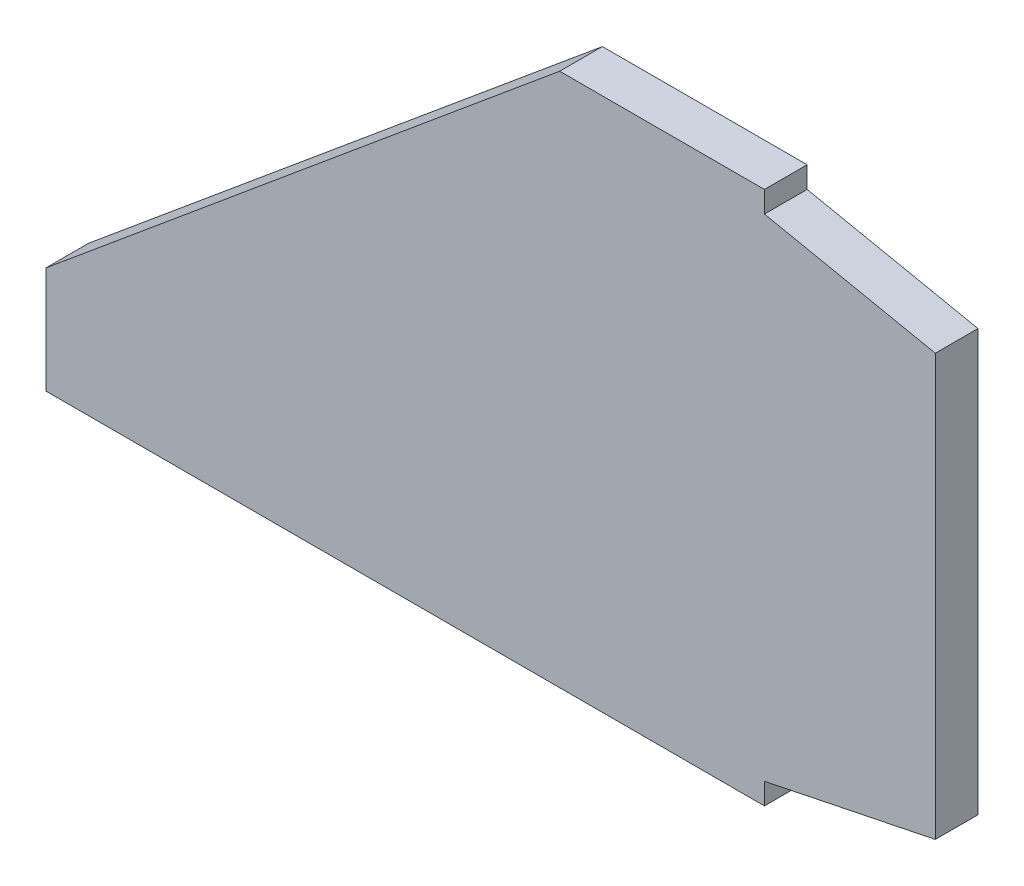
SolidWorks part; units mm, degrees
material "Q235B"
ref_plane "Front Plane" through (0, 0, 0) normal (0, 0, 1) x (1, 0, 0)
ref_plane "Top Plane" through (0, 0, 0) normal (0, 1, 0) x (1, 0, 0)
ref_plane "Right Plane" through (0, 0, 0) normal (1, 0, 0) x (0, 0, -1)
sketch "Sketch1" plane through (0, 0, 0) normal (0, 0, 1) x (1, 0, 0)
  line L0 (15783.13, 4624.3597) -> (15687.2573, 4624.3597)
  line L1 (15687.2573, 4624.3597) -> (15446.7284, 4424.3597)
  line L2 (15783.13, 4614.3597) -> (15783.13, 4624.3597)
  line L3 (15783.13, 4614.3597) -> (15863.13, 4597.9499)
  line L4 (15863.13, 4597.9499) -> (15863.13, 4400.7696)
  line L5 (15783.13, 4384.3597) -> (15863.13, 4400.7696)
  line L6 (15783.13, 4384.3597) -> (15783.13, 4374.3597)
  line L7 (15446.7284, 4374.3597) -> (15783.13, 4374.3597)
  line L8 (15446.7284, 4374.3597) -> (15446.7284, 4424.3597)
  dimension "D1" = 250
extrude "Boss-Extrude1" add sketch "Sketch1" along normal blind 20
